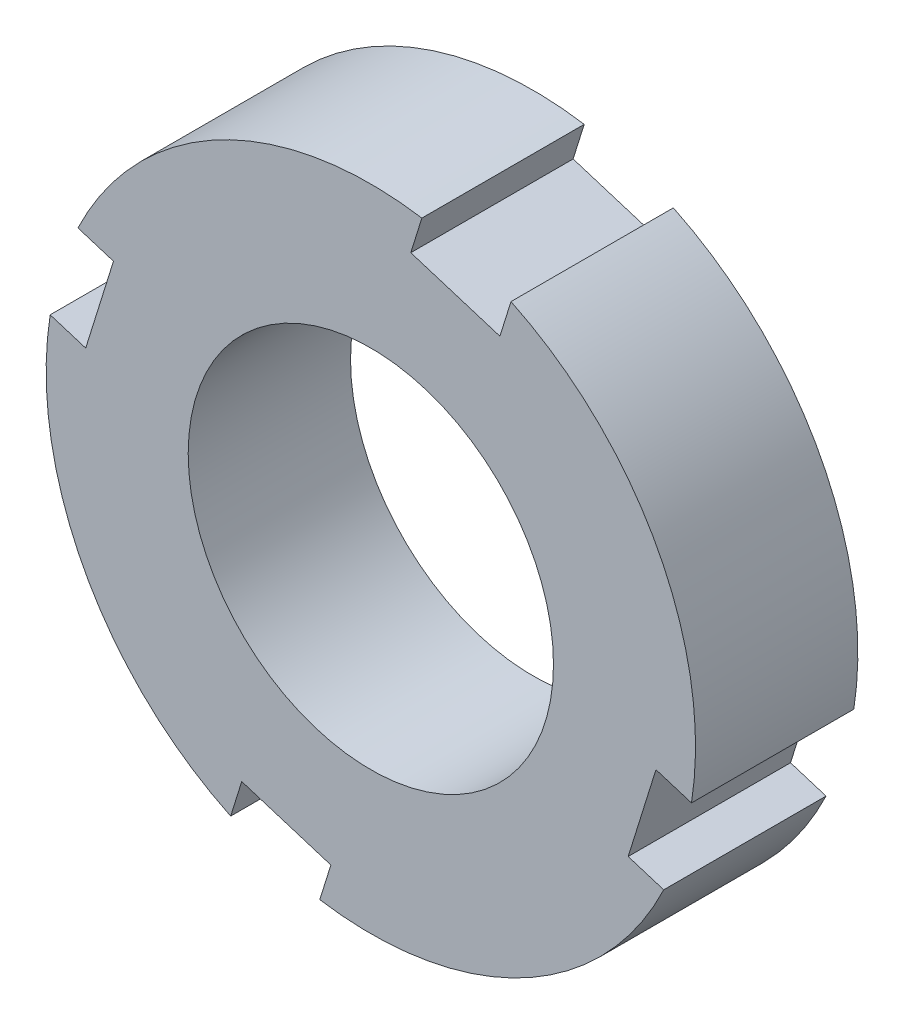
SolidWorks part; units mm, degrees
ref_plane "Front Plane" through (0, 0, 0) normal (0, 0, 1) x (1, 0, 0)
ref_plane "Top Plane" through (0, 0, 0) normal (0, 1, 0) x (1, 0, 0)
ref_plane "Right Plane" through (0, 0, 0) normal (1, 0, 0) x (0, 0, -1)
ref_plane "Plane1" through (0, 0, -1549.9984) normal (0, 0, 1) x (1, 0, 0)
sketch "Sketch1" plane through (0, 0, -1549.9984) normal (0, 0, 1) x (1, 0, 0)
  line L0 (526.154, 269.8698) -> (527.5179, 274.2467)
  line L1 (485.1493, 252.0105) -> (489.5262, 250.6465)
  line L2 (489.5262, 250.6465) -> (486.1048, 239.6673)
  line L3 (486.1048, 239.6673) -> (481.7279, 241.0313)
  line L4 (503.9641, 198.6626) -> (505.3281, 203.0395)
  line L5 (505.3281, 203.0395) -> (516.3073, 199.6181)
  line L6 (516.3073, 199.6181) -> (514.9434, 195.2412)
  line L7 (557.312, 217.4774) -> (552.9351, 218.8414)
  line L8 (552.9351, 218.8414) -> (556.3565, 229.8206)
  line L9 (556.3565, 229.8206) -> (560.7334, 228.4567)
  line L10 (538.4972, 270.8253) -> (537.1332, 266.4484)
  line L11 (537.1332, 266.4484) -> (526.154, 269.8698)
  arc A0 (527.5179, 274.2467) -> (485.1493, 252.0105) centre (521.2306, 234.744) ccw
  arc A1 (481.7279, 241.0313) -> (503.9641, 198.6626) centre (521.2306, 234.744) ccw
  arc A2 (514.9434, 195.2412) -> (557.312, 217.4774) centre (521.2306, 234.744) ccw
  arc A3 (560.7334, 228.4567) -> (538.4972, 270.8253) centre (521.2306, 234.744) ccw
  circle A4 centre (521.2306, 234.744) radius 22.5
  dimension "D1" = 45
  dimension "D2" = 40
  dimension "D3" = 40
  dimension "D4" = 40
  dimension "D5" = 40
  dimension "D6" = 3.4214
  dimension "D7" = 4.377
  dimension "D8" = 7.7984
  dimension "D9" = 22.2362
  dimension "D10" = 23.6002
  dimension "D11" = 33.2155
  dimension "D12" = 34.5795
  dimension "D13" = 39.5028
  dimension "D14" = 44.4261
  dimension "D15" = 45.7901
  dimension "D16" = 55.4054
  dimension "D17" = 56.7693
  dimension "D18" = 71.2072
  dimension "D19" = 74.6286
  dimension "D20" = 75.5842
  dimension "D21" = 79.0056
  dimension "D22" = 4.377
  dimension "D23" = 7.7984
  dimension "D24" = 23.6002
  dimension "D25" = 34.5795
  dimension "D26" = 44.4261
  dimension "D27" = 55.4054
  dimension "D28" = 71.2072
  dimension "D29" = 74.6286
extrude "Boss-Extrude1" add sketch "Sketch1" against normal blind 20
